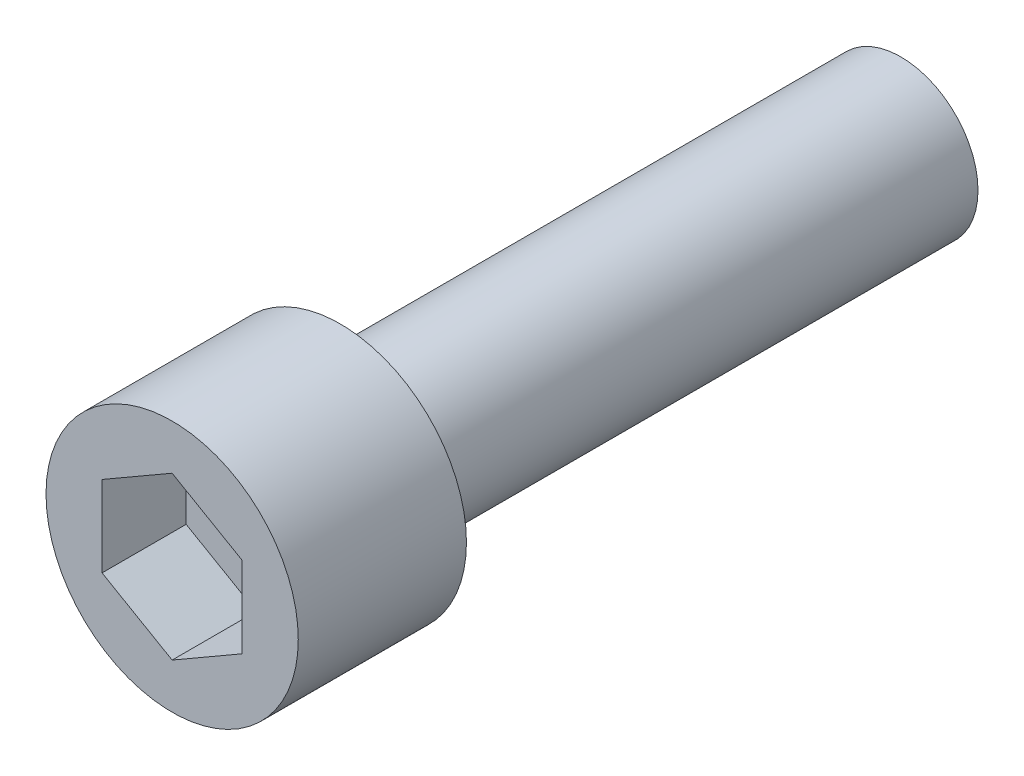
from build123d import *

# Parameters (mm, degrees)
SKETCH1_R           = 5.5
BOSS_EXTRUDE1_DEPTH = 40
SKETCH2_R           = 9
BOSS_EXTRUDE2_DEPTH = 12
CUT_EXTRUDE1_DEPTH  = 6


with BuildPart() as part:
    # Sketch1 → Boss-Extrude1 (new body)
    with BuildSketch(Plane.XY):
        Circle(SKETCH1_R)
    extrude(amount=BOSS_EXTRUDE1_DEPTH)

    # Sketch2 → Boss-Extrude2 (add)
    with BuildSketch(Plane.XY.offset(40)):
        Circle(SKETCH2_R)
    extrude(amount=BOSS_EXTRUDE2_DEPTH)

    # Sketch3 → Cut-Extrude1 (cut)
    with BuildSketch(Plane.XY.offset(52)):
        Polygon((0, 5.773502692), (-5, 2.886751346), (-5, -2.886751346), (0, -5.773502692), (5, -2.886751346), (5, 2.886751346), align=None)
    extrude(amount=-CUT_EXTRUDE1_DEPTH, mode=Mode.SUBTRACT)


solid = part.part
